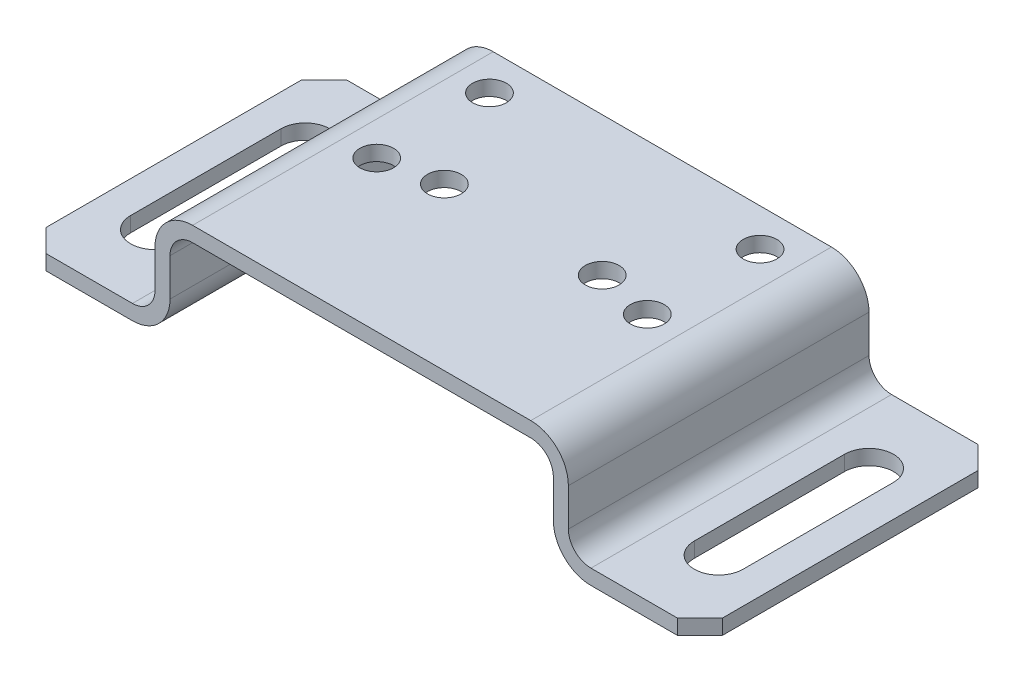
SolidWorks part; units mm, degrees
material "1023 碳钢板 (SS)"
ref_plane "前视基准面" through (0, 0, 0) normal (0, 0, 1) x (1, 0, 0)
ref_plane "上视基准面" through (0, 0, 0) normal (0, 1, 0) x (1, 0, 0)
ref_plane "右视基准面" through (0, 0, 0) normal (1, 0, 0) x (0, 0, -1)
sketch "草图2" plane through (0, 0, 0) normal (0, 0, 1) x (1, 0, 0)
  line L0 (0, 0) -> (14.5, 0)
  line L1 (17.5, 3) -> (17.5, 8)
  line L2 (22.5, 13) -> (67.5, 13)
  line L3 (72.5, 8) -> (72.5, 3)
  line L4 (75.5, 0) -> (90, 0)
  line L5 (0, -2) -> (14.5, -2)
  line L6 (19.5, 3) -> (19.5, 8)
  line L7 (22.5, 11) -> (67.5, 11)
  line L8 (70.5, 8) -> (70.5, 3)
  line L9 (75.5, -2) -> (90, -2)
  line L10 (0, 0) -> (0, -2)
  line L11 (90, 0) -> (90, -2)
  arc A0 (67.5, 13) -> (72.5, 8) centre (67.5, 8) cw
  arc A1 (17.5, 8) -> (22.5, 13) centre (22.5, 8) cw
  arc A2 (72.5, 3) -> (75.5, 0) centre (75.5, 3) ccw
  arc A3 (14.5, 0) -> (17.5, 3) centre (14.5, 3) ccw
  arc A4 (14.5, -2) -> (19.5, 3) centre (14.5, 3) ccw
  arc A5 (19.5, 8) -> (22.5, 11) centre (22.5, 8) cw
  arc A6 (67.5, 11) -> (70.5, 8) centre (67.5, 8) cw
  arc A7 (70.5, 3) -> (75.5, -2) centre (75.5, 3) ccw
  point P10 (72.5, 13)
  point P13 (17.5, 13)
  point P16 (72.5, 0)
  point P19 (17.5, 0)
  dimension "D5" = 5
  dimension "D6" = 3
  dimension "D1" = 17.5
  dimension "D2" = 55
  dimension "D3" = 17.5
  dimension "D4" = 13
  dimension "D7" = 2
extrude "凸台-拉伸1" add sketch "草图2" along normal blind 40 contours L11 L9 A7 L8 A6 L7 A5 L6 A4 L5 L10 L0 A3 L1 A1 L2 A0 L3 A2 L4
chamfer "倒角1" distance 3 angle 45 4 edges at (90, -1, 0) (90, -1, 40) (0, -1, 0) (0, -1, 40)
sketch "草图3" plane through (0, 0, 0) normal (0, 1, 0) x (1, 0, 0)
  line L0 (7.5, -10) -> (7.5, -30) construction
  line L1 (10.75, -10) -> (10.75, -30)
  line L2 (4.25, -10) -> (4.25, -30)
  line L3 (3, 0) -> (14.5, 0) construction
  line L4 (0, -37) -> (0, -3) construction
  line L5 (45, -40) -> (45, -17.8308)
  line L6 (22.5, -40) -> (67.5, -40) construction
  line L7 (82.5, -10) -> (82.5, -30) construction
  line L8 (79.25, -10) -> (79.25, -30)
  line L9 (85.75, -10) -> (85.75, -30)
  arc A0 (10.75, -10) -> (4.25, -10) centre (7.5, -10) ccw
  arc A1 (4.25, -30) -> (10.75, -30) centre (7.5, -30) ccw
  arc A2 (79.25, -10) -> (85.75, -10) centre (82.5, -10) cw
  arc A3 (85.75, -30) -> (79.25, -30) centre (82.5, -30) cw
  point P2 (7.5, -20)
  point P17 (82.5, -20)
  dimension "D1" = 10
  dimension "D2" = 20
  dimension "D3" = 6.5
  dimension "D4" = 7.5
extrude "切除-拉伸1" cut sketch "草图3" against normal blind 40 contours L2 A1 L1 A0 | A3 L9 A2 L8
sketch "草图4" plane through (0, 13, 0) normal (0, 1, 0) x (1, 0, 0)
  line L0 (45, 0) -> (45, -15.1993)
  line L1 (22.5, 0) -> (67.5, 0) construction
  circle A0 centre (27, -5) radius 2.25
  circle A1 centre (63, -5) radius 2.25
  circle A2 centre (34.5, -18.5) radius 2.25
  circle A3 centre (55.5, -18.5) radius 2.25
  circle A4 centre (27, -20) radius 2.25
  circle A5 centre (63, -20) radius 2.25
  point P12 (30.3539, -27.6165)
  point P13 (0, 0)
  point P14 (0, 0)
  dimension "D7" = 4.5
  dimension "D1" = 36
  dimension "D2" = 18
  dimension "D3" = 7.5
  dimension "D4" = 7.5
  dimension "D5" = 13.5
  dimension "D6" = 20
  dimension "D8" = 5
extrude "切除-拉伸2" cut sketch "草图4" against normal blind 40 contours A2 | A4 | A3 | A5 | A0 | A1
